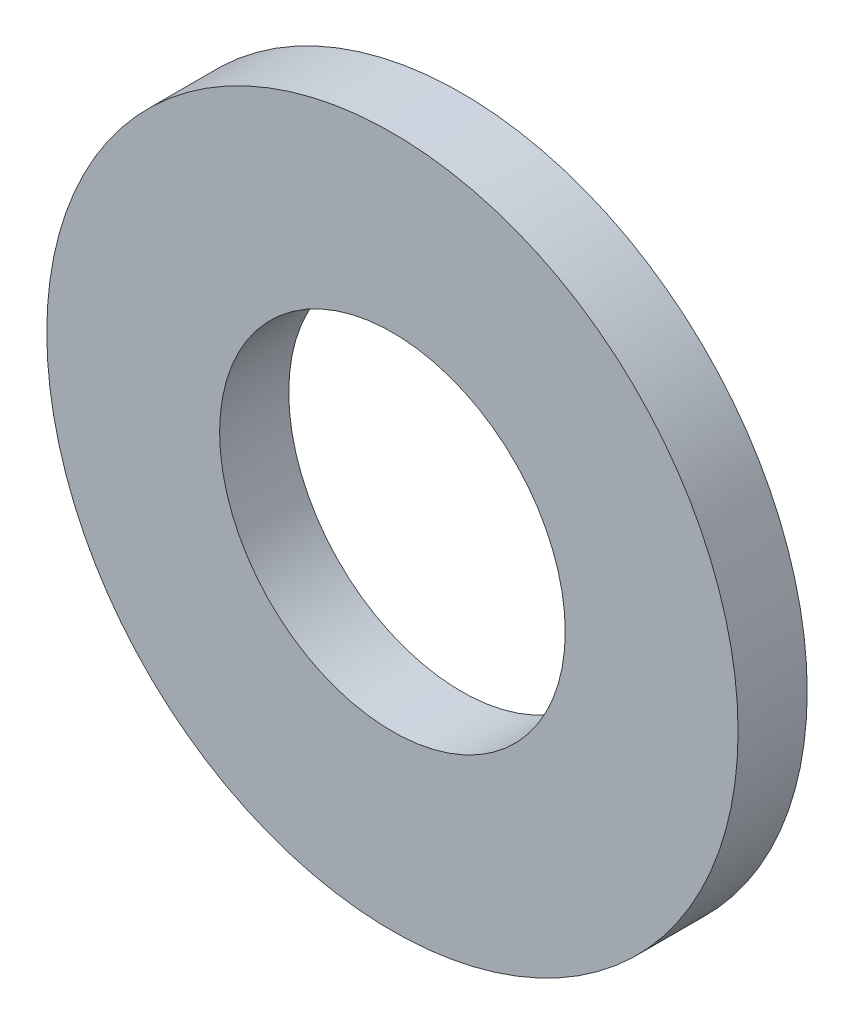
from build123d import *

# Parameters (mm, degrees)
SKETCH2_R           = 25
BOSS_EXTRUDE1_DEPTH = 2.5
SKETCH3_R           = 12.5
CUT_EXTRUDE1_DEPTH  = 108.470926301


with BuildPart() as part:
    # Sketch2 → Boss-Extrude1 (new, symmetric)
    with BuildSketch(Plane.XY):
        with Locations((-70, 25)):
            Circle(SKETCH2_R)
    extrude(amount=BOSS_EXTRUDE1_DEPTH, both=True)

    # Sketch3 → Cut-Extrude1 (cut, through all)
    with BuildSketch(Plane(origin=(0, 0, -2.5), x_dir=(-1, 0, 0), z_dir=(0, 0, -1))):
        with Locations((70, 25)):
            Circle(SKETCH3_R)
    extrude(amount=-CUT_EXTRUDE1_DEPTH, mode=Mode.SUBTRACT)


solid = part.part
